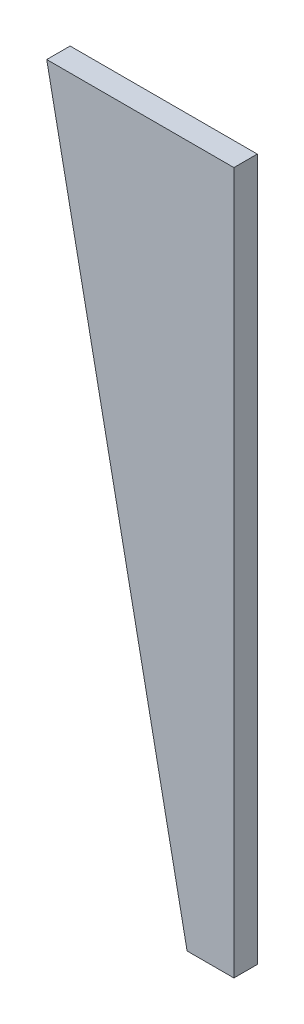
SolidWorks part; units mm, degrees
material "普通碳钢"
ref_plane "Front Plane" through (0, 0, 0) normal (0, 0, 1) x (1, 0, 0)
ref_plane "Top Plane" through (0, 0, 0) normal (0, 1, 0) x (1, 0, 0)
ref_plane "Right Plane" through (0, 0, 0) normal (1, 0, 0) x (0, 0, -1)
sketch "Sketch1" plane through (0, 0, 0) normal (0, 0, 1) x (1, 0, 0)
  line L0 (-80, 0) -> (0, 0)
  line L1 (0, 0) -> (0, -300)
  line L2 (0, -300) -> (-20, -300)
  line L3 (-20, -300) -> (-80, 0)
  dimension "D1" = 300
  dimension "D2" = 80
  dimension "D3" = 20
extrude "Extrude1" add sketch "Sketch1" along normal mid plane 10
